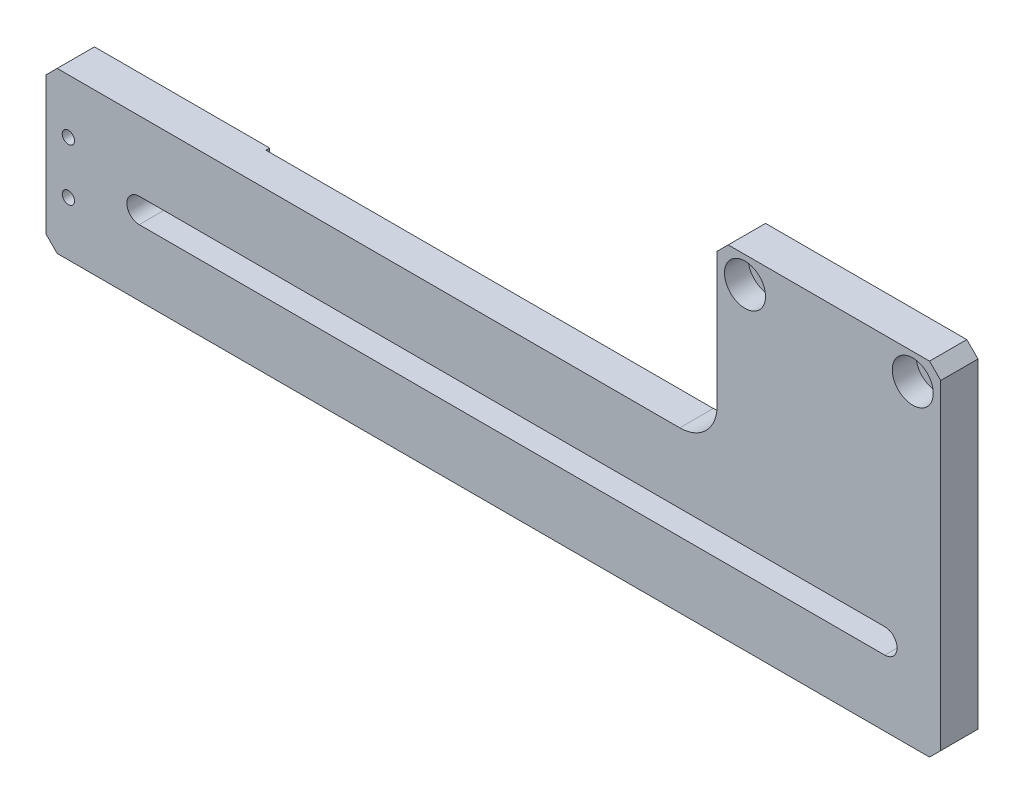
SolidWorks part; units mm, degrees
material "A6063"
ref_plane "Front Plane" through (0, 0, 0) normal (0, 0, 1) x (1, 0, 0)
ref_plane "Top Plane" through (0, 0, 0) normal (0, 1, 0) x (1, 0, 0)
ref_plane "Right Plane" through (0, 0, 0) normal (1, 0, 0) x (0, 0, -1)
sketch "Sketch1" plane through (0, 0, 0) normal (0, 0, 1) x (1, 0, 0)
  line L1 (-120, 46) -> (120, 46)
  line L2 (-120, 46) -> (-120, -46)
  line L3 (-120, -46) -> (120, -46)
  line L4 (120, 46) -> (120, -46)
  line L5 (-120, 46) -> (120, -46) construction
  line L6 (-120, -46) -> (120, 46) construction
  point P0 (0, 0)
  dimension "D1" = 240
  dimension "D2" = 92
extrude "Boss-Extrude1" add sketch "Sketch1" along normal blind 10
sketch "Sketch2" plane through (0, 0, 10) normal (0, 0, 1) x (1, 0, 0)
  line L0 (-95, -25) -> (105, -25) construction
  line L1 (-95, -21.7) -> (105, -21.7)
  line L2 (-95, -28.3) -> (105, -28.3)
  line L3 (-120, -46) -> (120, -46) construction
  line L4 (-120, 46) -> (-120, -46) construction
  arc A0 (-95, -21.7) -> (-95, -28.3) centre (-95, -25) ccw
  arc A1 (105, -28.3) -> (105, -21.7) centre (105, -25) ccw
  point P2 (5, -25)
  dimension "D1" = 21
  dimension "D2" = 25
  dimension "D3" = 200
  dimension "D4" = 6.6
extrude "Cut-Extrude1" cut sketch "Sketch2" against normal blind 10
sketch "Sketch3" plane through (0, 0, 10) normal (0, 0, 1) x (1, 0, 0)
  line L1 (-120, 46) -> (60, 46)
  line L2 (-120, 46) -> (-120, -3)
  line L3 (-120, -3) -> (60, -3)
  line L4 (60, 46) -> (60, -3)
  dimension "D1" = 180
  dimension "D2" = 49
extrude "Cut-Extrude2" cut sketch "Sketch3" against normal blind 10
fillet "Fillet1" radius 10 1 edges at (60, -3, 5)
chamfer "Chamfer1" distance 3 angle 45 5 edges at (-120, -46, 5) (-120, -3, 5) (120, -46, 5) (120, 46, 5) (60, 46, 5)
hole_wizard "M4 Tapped Hole1" positions "Sketch5" profile "Sketch4" tap size "M4" standard "Gb"
sketch "Sketch5" plane through (0, 0, 10) normal (0, 0, 1) x (1, 0, 0)
  line L0 (-120, -24.5) -> (-88.2005, -24.5) construction
  line L1 (-120, -6) -> (-120, -43) construction
  point P0 (-114, -17.5)
  point P3 (-114, -31.5)
  dimension "D1" = 6
  dimension "D2" = 14
sketch "Sketch4" plane through (-114, -17.5, 10) normal (1, 0, 0) x (0, -1, 0)
  line L0 (0, 0) -> (0, 12.4914)
  line L1 (0, 12.4914) -> (1.65, 11.5)
  line L2 (1.65, 11.5) -> (1.65, 0)
  line L5 (1.65, 0) -> (0, 0)
  line L10 (0, 12.4914) -> (-1.65, 11.5) construction
  line L11 (0, -6.35) -> (0, 107.95) construction
  dimension "螺纹孔钻头直径" = 3.3
  dimension "螺纹孔钻头深度" = 11.5
  dimension "导头角度" = 118
cosmetic thread "Cosmetic thread 1" parameters "D1"=8, "D2"=4
cosmetic thread "Cosmetic thread 2" parameters "D1"=8, "D2"=4
hole_wizard "CBORE for M6 Hex Socket Head Cap Screw1" positions "Sketch7" profile "Sketch6" counterbore size "M6" standard "Iso" end condition through all
sketch "Sketch7" plane through (0, 0, 10) normal (0, 0, 1) x (1, 0, 0)
  line L3 (90, 46) -> (90, 10.2426) construction
  line L4 (117, 46) -> (63, 46) construction
  point P0 (67.5, 39)
  point P2 (112.5, 39)
  dimension "D1" = 45
  dimension "D2" = 7
sketch "Sketch6" plane through (67.5, 39, 10) normal (1, 0, 0) x (0, -1, 0)
  line L0 (0, 0) -> (0, 10)
  line L1 (0, 10) -> (3.2, 10)
  line L3 (3.2, 10) -> (3.2, 6.4)
  line L4 (3.2, 6.4) -> (5.5, 6.4)
  line L5 (5.5, 6.4) -> (5.5, 0)
  line L7 (5.5, 0) -> (0, 0)
  line L11 (0, -6.35) -> (0, 107.95) construction
  dimension "通孔孔直径" = 6.4
  dimension "通孔孔深度" = 10
  dimension "柱形沉头孔直径" = 11
  dimension "柱形沉头孔深度" = 6.4
sketch "Sketch8" plane through (0, 0, 0) normal (0, 0, -1) x (-1, 0, 0)
  line L0 (117, -46) -> (-117, -46) construction
  line L1 (70, -46) -> (-60, -46)
  line L2 (70, -46) -> (70, 43)
  line L3 (70, 43) -> (-60, 43)
  line L4 (-60, -46) -> (-60, 43)
  line L5 (120, -6) -> (120, -43) construction
  dimension "D1" = 50
extrude "Cut-Extrude3" cut sketch "Sketch8" against normal blind 1
